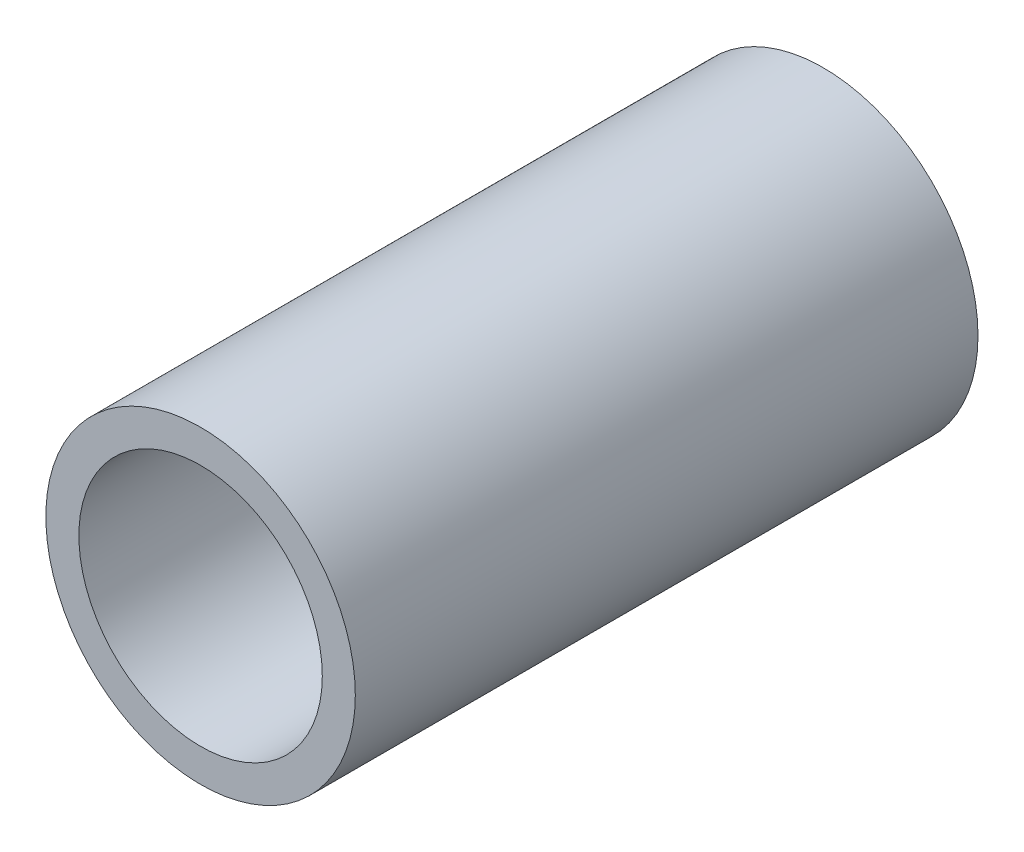
from build123d import *

# Parameters (mm, degrees)
SKETCH1_R           = 41.25
SKETCH1_R_2         = 32.45
BOSS_EXTRUDE1_DEPTH = 166


with BuildPart() as part:
    # Sketch1 → Boss-Extrude1 (new body)
    with BuildSketch(Plane.XY):
        Circle(SKETCH1_R)
        Circle(SKETCH1_R_2, mode=Mode.SUBTRACT)
    extrude(amount=BOSS_EXTRUDE1_DEPTH)


solid = part.part
